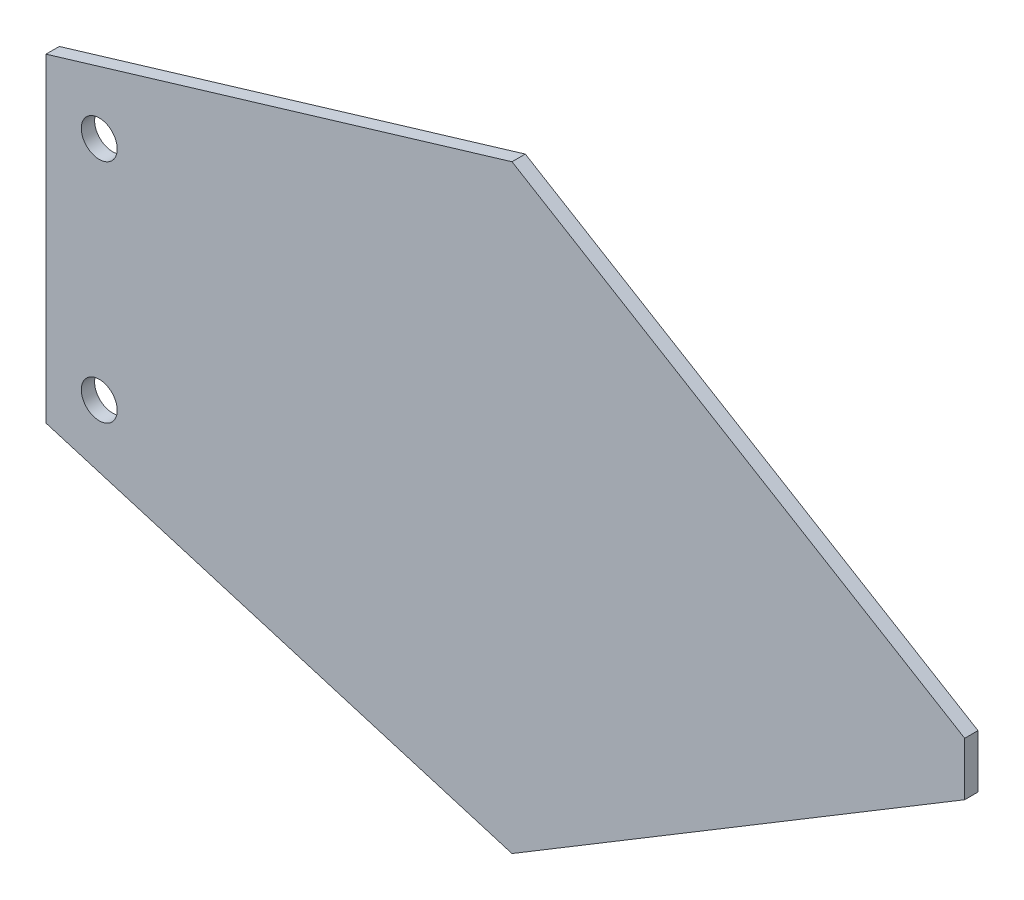
SolidWorks part; units mm, degrees
material "1023 碳钢板 (SS)"
ref_plane "前视基准面" through (0, 0, 0) normal (0, 0, 1) x (1, 0, 0)
ref_plane "上视基准面" through (0, 0, 0) normal (0, 1, 0) x (1, 0, 0)
ref_plane "右视基准面" through (0, 0, 0) normal (1, 0, 0) x (0, 0, -1)
sketch "草图1" plane through (0, 0, 0) normal (0, 0, 1) x (1, 0, 0)
  line L1 (345, -225) -> (-345, -225)
  line L2 (345, -225) -> (345, 225)
  line L3 (345, 225) -> (-345, 225)
  line L4 (-345, -225) -> (-345, 225)
  line L5 (345, -225) -> (-345, 225) construction
  line L6 (345, 225) -> (-345, -225) construction
  point P0 (0, 0)
  dimension "D1" = 690
  dimension "D2" = 450
extrude "凸台-拉伸1" add sketch "草图1" along normal blind 10
sketch "草图2" plane through (0, 0, 10) normal (0, 0, 1) x (1, 0, 0)
  line L0 (-345, -120) -> (5, -225)
  line L1 (-345, 225) -> (-345, -225) construction
  line L3 (5, -225) -> (-345, -225)
  line L4 (-345, -225) -> (-345, -120)
  line L6 (5, 225) -> (-345, 225)
  line L7 (-345, 120) -> (5, 225)
  line L8 (-345, 225) -> (-345, 120)
  line L9 (5, 225) -> (345, 20)
  line L10 (345, 225) -> (-345, 225) construction
  line L11 (345, -225) -> (345, 225) construction
  line L12 (345, 20) -> (345, 225)
  line L13 (345, 225) -> (5, 225)
  line L14 (345, -20) -> (345, -225)
  line L15 (5, -225) -> (345, -20)
  line L16 (345, -225) -> (5, -225)
  circle A0 centre (-305, -85) radius 13.5
  circle A1 centre (-305, 85) radius 13.5
  line M1 (-345, 225) -> (-345, -225)
  line M2 (-345, -225) -> (345, -225)
  line M3 (345, -225) -> (345, 225)
  line M4 (345, 225) -> (-345, 225)
  dimension "D4" = 27
  dimension "D6" = 40
  dimension "D1" = 105
  dimension "D3" = 170
  dimension "D7" = 205
  dimension "D8" = 340
extrude "切除-拉伸1" cut sketch "草图2" against normal blind 10 contours L7 M1 M4 | L9 M4 M3 | L15 M2 M3 | L0 M1 M2 | A0 | A1
